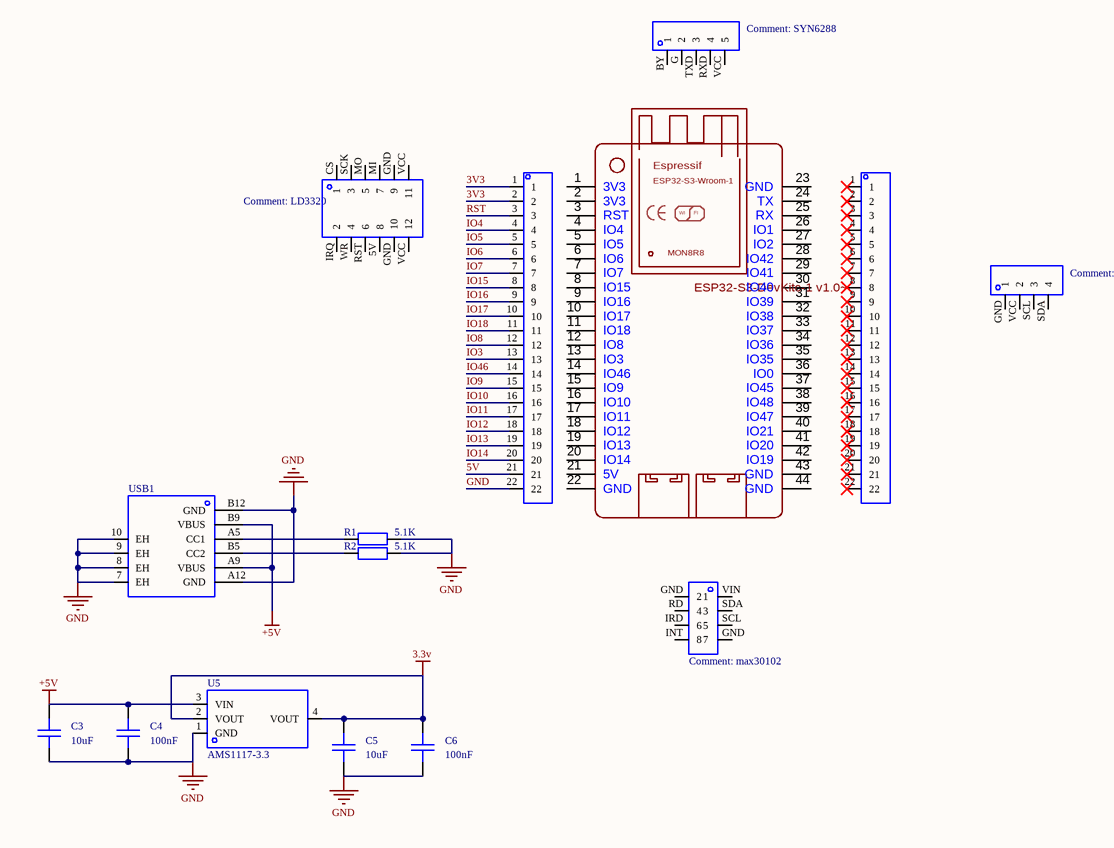
[diagram p0: MISC49904-3.schdoc]
# Altium project MISC49904-2.PrjPcb
1 sheet, 15 parts. Net scope: global (net labels, ports and power ports of the same name join across sheets).
Board file: MISC49904.pcbdoc

## Sheet MISC49904-3.schdoc
size 297 x 209 mm; Version: V1.0; @Project Name: MISC49904; @Update Date: 2026-04-21; @Create Date: 2026-04-21; @Board Name: MISC49904; @Create Time: 16:58:48; @Page Count: 1; @Page No: 1; @Schematic Name: MISC49904; @Update Time: 16:58:48; Size: A4

### Parts
C3  10uF  [C0603]
C4  100nF  [C0603]
C5  10uF  [C0603]
C6  100nF  [C0603]
H1  CS-1165SDIG-1*22  [HDR-TH_22P-P2.54-V-F]  (value not drawn)
H2  CS-1165SDIG-1*22  [HDR-TH_22P-P2.54-V-F]  (value not drawn)
H3  LD3320  [HDR-TH_12P-P2.54-V-F-R2-C6-S2.54]
H4  SYN6288  [HDR-TH_5P-P2.54-V-F]
H5  OLED  [HDR-TH_4P-P2.54-V-F]
R1  5.1K  [R0603]
R2  5.1K  [R0603]
U1  ESP32-S3-DEVKITC-1-1000MIL  [ESP32-S3-DEVKITC-1-1000MIL]  (value not drawn)
U2  max30102  [HDR-TH_8P-P2.54-V-F-R2-C4-S2.54]
U5  AMS1117-3.3  [SOT-223-3_L6.5-W3.4-P2.30-LS7.0-BR]
USB1  (no value)  [USB_ TYPE-C-6P]

### Nets
3.3v: C5.2 C6.2 U5.2(VOUT) U5.4(VOUT)
+5V: C3.2 C4.2 U5.3(VIN) USB1.A9(VBUS) USB1.B9(VBUS)
GND: C3.1 C4.1 C5.1 C6.1 H1.22 R1.2 R2.2 U5.1(GND) USB1.7(EH) USB1.8(EH) USB1.9(EH) USB1.10(EH) USB1.A12(GND) USB1.B12(GND)
3V3: H1.1 H1.2
5V: H1.21
IO3: H1.13
IO4: H1.4
IO5: H1.5
IO6: H1.6
IO7: H1.7
IO8: H1.12
IO9: H1.15
IO10: H1.16
IO11: H1.17
IO12: H1.18
IO13: H1.19
IO14: H1.20
IO15: H1.8
IO16: H1.9
IO17: H1.10
IO18: H1.11
IO46: H1.14
RST: H1.3
NetR1_1: R1.1 USB1.A5(CC1)
NetR2_1: R2.1 USB1.B5(CC2)

Not connected (* = marked no-connect by the designer): H2 1* 2* 3* 4* 5* 6* 7* 8* 9* 10* 11* 12* 13* 14* 15* 16* 17* 18* 19* 20* 21* 22*; H3 5V(8) CS(1) GND(10) IRQ(2) MI(7) MO(5) RST(6) SCK(3) VCC(12) WR(4); H4 BY(1) G(2) RXD(4) TXD(3) VCC(5); H5 GND(1) SCL(3) SDA(4) VCC(2); U1 1(3V3) 2(3V3) 3(RST) 4(IO4) 5(IO5) 6(IO6) 7(IO7) 8(IO15) 9(IO16) 10(IO17) 11(IO18) 12(IO8) 13(IO3) 14(IO46) 15(IO9) 16(IO10) 17(IO11) 18(IO12) 19(IO13) 20(IO14) 21(5V) 22(GND) 23(GND) 24(TX) 25(RX) 26(IO1) 27(IO2) 28(IO42) 29(IO41) 30(IO40) 31(IO39) 32(IO38) 33(IO37) 34(IO36) 35(IO35) 36(IO0) 37(IO45) 38(IO48) 39(IO47) 40(IO21) 41(IO20) 42(IO19) 43(GND) 44(GND); U2 GND(7) INT(8) IRD(6) RD(4) SCL(5) SDA(3) VIN(1)

### Notes on the sheet
- 2026-04-21
- 原理图
- P1
- 1.0
- 版本
- 尺寸
- A4
- 页    1    共    1

### Library data of the parts
C3-C6 = CAP_0603: Symbol: Capacitance; 3D Model: ac125912035d415993ca9572d50418b10819f05c4eef4c71ace90d822a990e87; 3D Model Transform: 62.992,31.496,0,0,0,0,0,0,0; ConvertToPcb: yes; ModelName: C0603_L1.6-W0.8-H0.8; Device: CAP_0603; Supplier Footprint: 0603; AddInBom: yes; FootprintName: C0603
  C3 C5: Value: 10uF
  C4 C6: Value: 100nF
H1 H2 = CS-1165SDIG-1*22: 插孔结构:1x22P;间距:2.54mm;行距:-;圆孔/方孔:方孔;安装方式:直插;排数:单排;总孔位数:22P;额定电流:3A;额定电压:250V;插孔方向:顶部;塑高:8.5mm;工作温度:-40℃~+105℃;; Manufacturer: CST(永丰盈); AddInBom: yes; ModelId: 0181345c91514c0db21026e9170582810819f05c4eef4c71ace90d822a990e87; ModelTransform: 2199.99552,98.425,0,0,0,0,0,0,-125.984; Holes Structure: 1x22P; Pitch: 2.54mm; Circular Hole / Square Hole: 方孔; Number of Positions: 22P; Current Rating: 3A; Voltage Rating (Max): 250V; Holes Direction: 顶部; Symbol: CS-1165SDIG-1*22; Device: CS-1165SDIG-1*22; LCSC Part Name: 间距:2.54mm 1x22P 直插; SupplierPart: C2886702; ManufacturerPart: CS-1165SDIG-1*22; Supplier Footprint: 插件,P=2.54mm; JLCPCB Part Class: Extended Part; Datasheet: https://item.szlcsc.com/datasheet/CS-1165SDIG-1*22/3101052.html; Supplier: LCSC; ConvertToPcb: yes; FootprintName: HDR-TH_22P-P2.54-V-F; ModelName: HDR-TH_22P-P2.54-V-F; Row Spacing: -; Mounting Type: 直插; Number of Rows: 单排; Insulation Height: 8.5mm; Operating Temperature: -40℃~+105℃
H3 = PM254V-12-12-H85: 插孔结构:2x6P;间距:2.54mm;行距:2.54mm;圆孔/方孔:方孔;安装方式:直插;排数:双排;总孔位数:12P;额定电流:3A;额定电压:250V;插孔方向:顶部;塑高:8.5mm;触头材质:黄铜;触头镀层:-;工作温度:-40℃~+105℃;; Manufacturer: XFCN(兴飞); AddInBom: yes; ModelId: 95d1f1a5666d46438f9c767a173340ed0819f05c4eef4c71ace90d822a990e87; ModelName: HDR-TH_12P-P2.54-F-LI-2X6P; ModelTransform: 615.7468,196.85,0,0,0,0,0,0,-129.921; Holes Structure: 2x6P; Pitch: 2.54mm; Circular Hole / Square Hole: 方孔; Number of Positions: 12P; Current Rating: 3A; Voltage Rating (Max): 250V; Holes Direction: 顶部; Symbol: PM254V-12-12-H85; Device: PM254V-12-12-H85; LCSC Part Name: 2x6P 间距:2.54mm 直插; SupplierPart: C541855; ManufacturerPart: PM254V-12-12-H85; Supplier Footprint: 插件,P=2.54mm; JLCPCB Part Class: Extended Part; Datasheet: https://item.szlcsc.com/datasheet/PM254V-12-12-H85/562476.html; Supplier: LCSC; ConvertToPcb: yes; FootprintName: HDR-TH_12P-P2.54-V-F-R2-C6-S2.54; Row Spacing: 2.54mm; Mounting Type: 直插; Number of Rows: 双排; Insulation Height: 8.5mm; Contact Material: 黄铜; Contact Plating: -; Operating Temperature: -40℃~+105℃
H4 = PM254V-11-05-H85: 插孔结构:1x5P;间距:2.54mm;行距:-;圆孔/方孔:方孔;安装方式:直插;排数:单排;总孔位数:5P;额定电流:3A;插孔方向:顶部;塑高:8.5mm;触头材质:黄铜;触头镀层:-;工作温度:-40℃~+105℃;; Manufacturer: XFCN(兴飞); AddInBom: yes; ModelId: f49cb6116a3d45e5a64915bf3e00773f0819f05c4eef4c71ace90d822a990e87; ModelTransform: 519.684,98.464,0,0,0,0,0,0,-124.016; Holes Structure: 1x5P; Pitch: 2.54mm; Circular Hole / Square Hole: 方孔; Number of Positions: 5P; Current Rating: 3A; Holes Direction: 顶部; Symbol: PM254V-11-05-H85; Device: PM254V-11-05-H85; LCSC Part Name: 1x5P 间距:2.54mm 直插; SupplierPart: C541852; ManufacturerPart: PM254V-11-05-H85; Supplier Footprint: 插件,P=2.54mm; JLCPCB Part Class: Extended Part; Datasheet: https://item.szlcsc.com/datasheet/PM254V-11-05-H85/562473.html; Supplier: LCSC; ConvertToPcb: yes; FootprintName: HDR-TH_5P-P2.54-V-F; ModelName: HDR-TH_5P-P2.54-V-F; Row Spacing: -; Mounting Type: 直插; Number of Rows: 单排; Insulation Height: 8.5mm; Contact Material: 黄铜; Contact Plating: -; Operating Temperature: -40℃~+105℃
H5 = 2.54-1*4P母: 插孔结构:1x4P;间距:2.54mm;行距:-;圆孔/方孔:方孔;安装方式:直插;排数:单排;总孔位数:4P;额定电流:3A;额定电压:-;插孔方向:顶部;塑高:-;触头材质:青铜;触头镀层:-;工作温度:-40℃~+105℃;; Manufacturer: BOOMELE(博穆精密); AddInBom: yes; ModelId: d187812051054f85879fcaa51a310d8e0819f05c4eef4c71ace90d822a990e87; ModelTransform: 419.6842,98.464,0,0,0,0,0,0,-118.11; Holes Structure: 1x4P; Pitch: 2.54mm; Circular Hole / Square Hole: 方孔; Number of Positions: 4P; Current Rating: 3A; Holes Direction: 顶部; Symbol: 2.54-1*4P母; Device: 2.54-1*4P母; LCSC Part Name: 间距:2.54mm 1x4P 直插; SupplierPart: C2718488; ManufacturerPart: 2.54-1*4P母; Supplier Footprint: 插件,P=2.54mm; JLCPCB Part Class: Extended Part; Datasheet: https://item.szlcsc.com/datasheet/2.54-1*4P%25E6%25AF%258D/2834502.html; Supplier: LCSC; ConvertToPcb: yes; FootprintName: HDR-TH_4P-P2.54-V-F; ModelName: HDR-TH_4P-P2.54-V-F; Row Spacing: -; Mounting Type: 直插; Number of Rows: 单排; Voltage Rating (Max): -; Insulation Height: -; Contact Material: 青铜; Contact Plating: -; Operating Temperature: -40℃~+105℃
R1 R2 = Res_0603: Symbol: 电阻; ConvertToPcb: yes; ModelId: fc143cca1e79419f9cd78b61e9279f080819f05c4eef4c71ace90d822a990e87; ModelTransform: 31.8897,63.7794,0,90,0,0,0,0,0; Device: Res_0603; Value: 5.1K; AddInBom: yes; Supplier Footprint: 0603; FootprintName: R0603; ModelName: R0603
U1 = ESP32-S3-DEVKITC-1-1000MIL: ESP32-S3-DevKitC-1; Manufacturer: 乐鑫科技; Symbol: ESP32-S3-DEVKITC-1-1000MIL; Device: ESP32-S3-DEVKITC-1-1000MIL; ManufacturerPart: ESP32-S3; Supplier: 乐鑫科技; SupplierPart: ESP32-S3; link: https://www.espressif.com/zh-hans/products/socs/esp32-s3; FootprintName: ESP32-S3-DEVKITC-1-1000MIL
U2 = PM254-2-04-Z-8.5: 插孔结构:2x4P;间距:2.54mm;行距:2.54mm;圆孔/方孔:方孔;安装方式:直插;排数:双排;总孔位数:8P;额定电流:3A;额定电压:-;插孔方向:顶部;塑高:8.5mm;触头材质:铜合金;工作温度:-40℃~+105℃;; Manufacturer: HCTL(华灿天禄); AddInBom: yes; ModelId: 52f9c7b3691648c0a1959c61eae445900819f05c4eef4c71ace90d822a990e87; ModelName: HDR-TH_8P-P2.54-F-LI-2X4P; ModelTransform: 415.7472,196.85,0,0,0,0,0,0,-118.11; Holes Structure: 2x4P; Pitch: 2.54mm; Circular Hole / Square Hole: 方孔; Number of Positions: 8P; Current Rating: 3A; Holes Direction: 顶部; Symbol: PM254-2-04-Z-8.5; Device: PM254-2-04-Z-8.5; LCSC Part Name: 2x4P 间距:2.54mm 直插; SupplierPart: C2897405; ManufacturerPart: PM254-2-04-Z-8.5; Supplier Footprint: 插件,P=2.54mm; JLCPCB Part Class: Extended Part; Datasheet: https://item.szlcsc.com/datasheet/PM254-2-04-Z-8.5/3142410.html; Supplier: LCSC; ConvertToPcb: yes; FootprintName: HDR-TH_8P-P2.54-V-F-R2-C4-S2.54; Row Spacing: 2.54mm; Mounting Type: 直插; Number of Rows: 双排; Voltage Rating (Max): -; Insulation Height: 8.5mm; Contact Material: 铜合金; Operating Temperature: -40℃~+105℃
U5 = AMS1117-3.3_C6186: 输出类型:固定;工作电压:15V;输出电压:3.3V;输出电流:1A;电源纹波抑制比(PSRR):72dB@(120Hz);输出极性:正极;; Manufacturer: AMS; AddInBom: yes; ModelId: 925194bf9823436183a3e0b978a8d0760819f05c4eef4c71ace90d822a990e87; ModelName: SOT-223-4P_L6.5-W3.5-H1.6-LS7.0-P2.30; ModelTransform: 279.89794,255.905,0,180,0,0,-3.9385,-0.0005,0; Output Type: 固定; Voltage - Supply: 15V; Output Voltage: 3.3V; Output Current: 1A; Voltage Dropout: 1.1V@(800mA); standby current: 5mA; Noise: 0.003%Vout; Output Configuration: 正极; Number of Outputs: 1; Symbol: AMS1117-3.3; Device: AMS1117-3.3_C6186; LCSC Part Name: 3.3V 1A 15V; SupplierPart: C6186; ManufacturerPart: AMS1117-3.3; Supplier Footprint: SOT-223; JLCPCB Part Class: Basic Part; Datasheet: https://item.szlcsc.com/datasheet/AMS1117-3.3/6652.html; Supplier: LCSC; ConvertToPcb: yes; FootprintName: SOT-223-3_L6.5-W3.4-P2.30-LS7.0-BR; Power Supply Rejection Ratio (PSRR): 72dB@(120Hz); Features: 过流保护；热关断; Operating Temperature: -40℃~+125℃
USB1 = USB_ Type-C-6P: AddInBom: yes; ModelId: d4f492a4e6024845a13b3f6a4ef2d2cb0819f05c4eef4c71ace90d822a990e87; ModelName: USB-SMD_U262-061N-4BVC11; ModelTransform: 352.362,281.496,0,0,0,0,0,-47.244,-39.37; Symbol: USB_ TYPE-C-6P; Device: USB_ Type-C-6P; Supplier Footprint: SMD; ConvertToPcb: yes; FootprintName: USB_ TYPE-C-6P